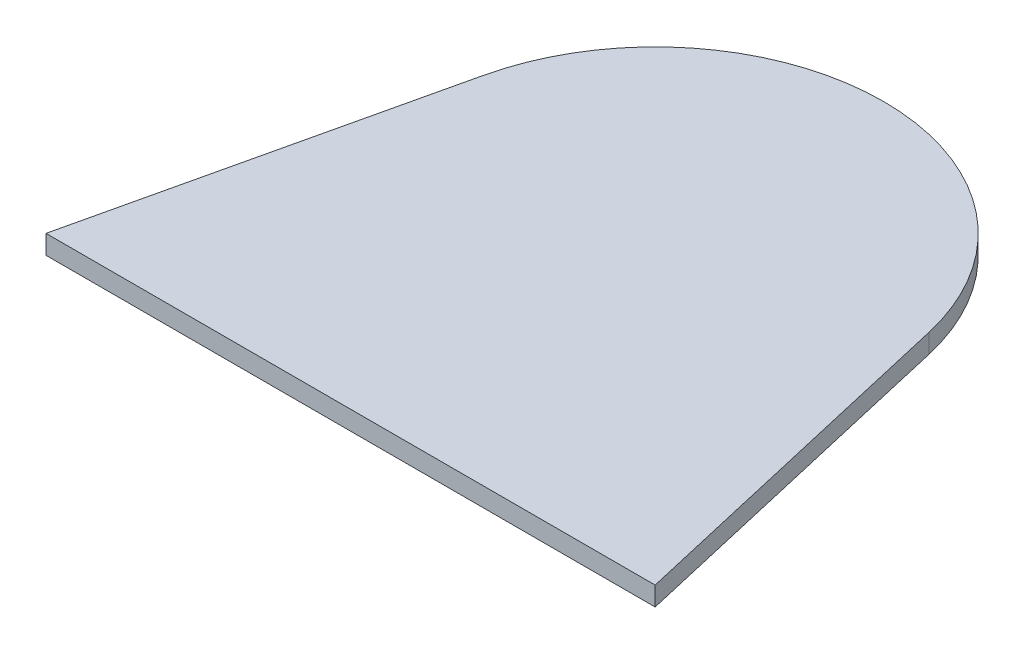
SolidWorks part; units mm, degrees
material "A3"
ref_plane "前视基准面" through (0, 0, 0) normal (0, 0, 1) x (1, 0, 0)
ref_plane "上视基准面" through (0, 0, 0) normal (0, 1, 0) x (1, 0, 0)
ref_plane "右视基准面" through (0, 0, 0) normal (1, 0, 0) x (0, 0, -1)
sketch "草图1" plane through (0, 0, 0) normal (0, 1, 0) x (1, 0, 0)
  line L0 (0, 0) -> (0, -80) construction
  line L1 (80, -80) -> (-80, -80)
  line L2 (-80, -80) -> (-58.4687, 13.4687)
  line L3 (80, -80) -> (58.4687, 13.4687)
  arc A0 (58.4687, 13.4687) -> (-58.4687, 13.4687) centre (0, 0) ccw
  dimension "D1" = 120
  dimension "D2" = 160
  dimension "D3" = 80
extrude "凸台-拉伸1" add sketch "草图1" along normal blind 5
